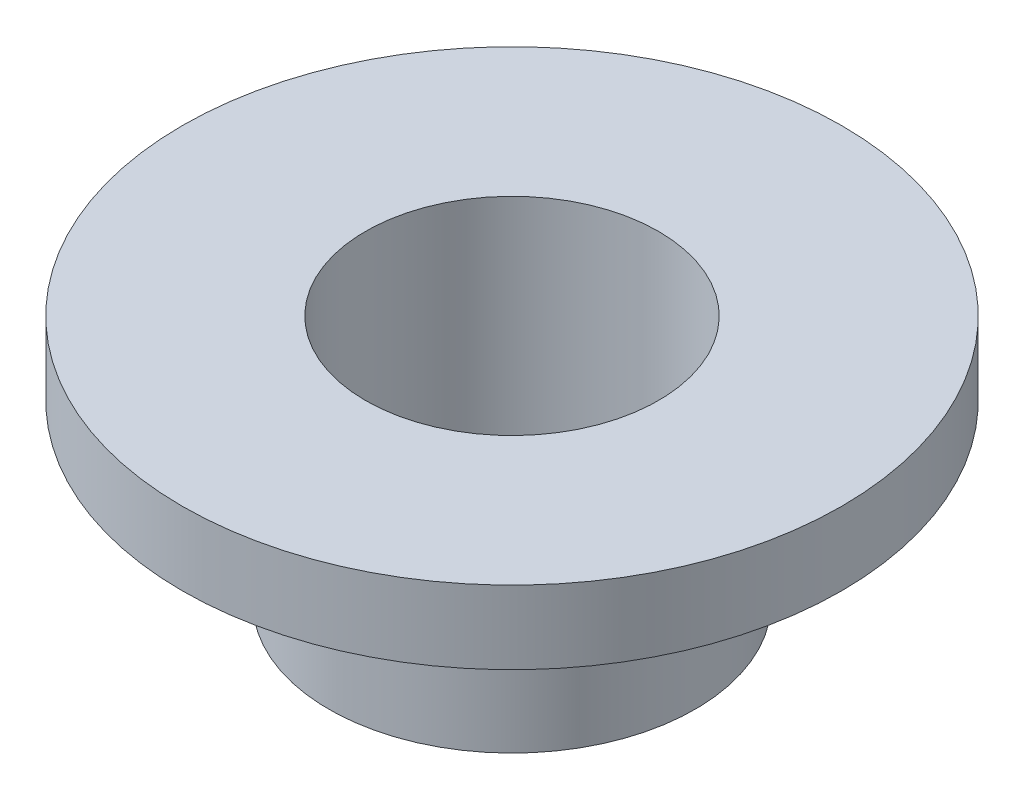
SolidWorks part; units mm, degrees
material "T3"
ref_plane "前视基准面" through (0, 0, 0) normal (0, 0, 1) x (1, 0, 0)
ref_plane "上视基准面" through (0, 0, 0) normal (0, 1, 0) x (1, 0, 0)
ref_plane "右视基准面" through (0, 0, 0) normal (1, 0, 0) x (0, 0, -1)
sketch "草图1" plane through (0, 0, 0) normal (0, 0, 1) x (1, 0, 0)
  line L0 (0, 0) -> (0, 19.9287) construction
  line L1 (0, 0) -> (22.5, 0)
  line L2 (22.5, 0) -> (22.5, -5)
  line L3 (22.5, -5) -> (12.5, -5)
  line L4 (12.5, -5) -> (12.5, -17)
  line L5 (12.5, -17) -> (0, -17)
  line L6 (0, -17) -> (0, 0)
  dimension "D1" = 5
  dimension "D2" = 45
  dimension "D3" = 17
  dimension "D4" = 12.5
revolve "旋转1" add sketch "草图1" angle 360 about L0
sketch "草图2" plane through (0, -17, 0) normal (0, -1, 0) x (1, 0, 0)
  circle A0 centre (0, 0) radius 10
  dimension "D1" = 20
extrude "切除-拉伸1" cut sketch "草图2" against normal blind 26
